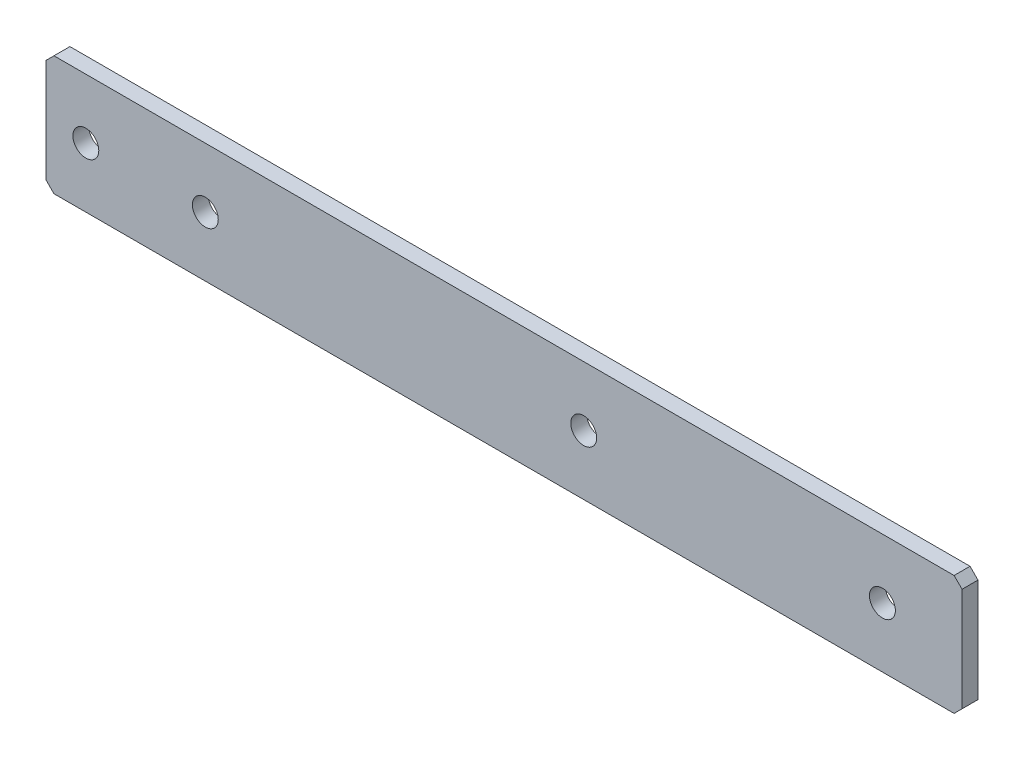
SolidWorks part; units mm, degrees
material "1023 碳钢板 (SS)"
ref_plane "Front Plane" through (0, 0, 0) normal (0, 0, 1) x (1, 0, 0)
ref_plane "Top Plane" through (0, 0, 0) normal (0, 1, 0) x (1, 0, 0)
ref_plane "Right Plane" through (0, 0, 0) normal (1, 0, 0) x (0, 0, -1)
sketch "Sketch1" plane through (0, 0, 0) normal (0, 0, 1) x (1, 0, 0)
  line L1 (115, 15) -> (-115, 15)
  line L2 (115, 15) -> (115, -15)
  line L3 (115, -15) -> (-115, -15)
  line L4 (-115, 15) -> (-115, -15)
  line L5 (115, 15) -> (-115, -15) construction
  line L6 (115, -15) -> (-115, 15) construction
  circle A0 centre (-105, 0) radius 3.25
  circle A1 centre (-75, 0) radius 3.25
  circle A2 centre (20, 0) radius 3.25
  circle A3 centre (95, 0) radius 3.25
  point P0 (0, 0)
  dimension "D3" = 10
  dimension "D4" = 30
  dimension "D5" = 95
  dimension "D6" = 6.5
  dimension "D7" = 75
  dimension "D1" = 30
  dimension "D2" = 230
extrude "Boss-Extrude1" add sketch "Sketch1" along normal blind 4
chamfer "Chamfer1" distance 2 angle 45 4 edges at (-115, -15, 2) (-115, 15, 2) (115, -15, 2) (115, 15, 2)
